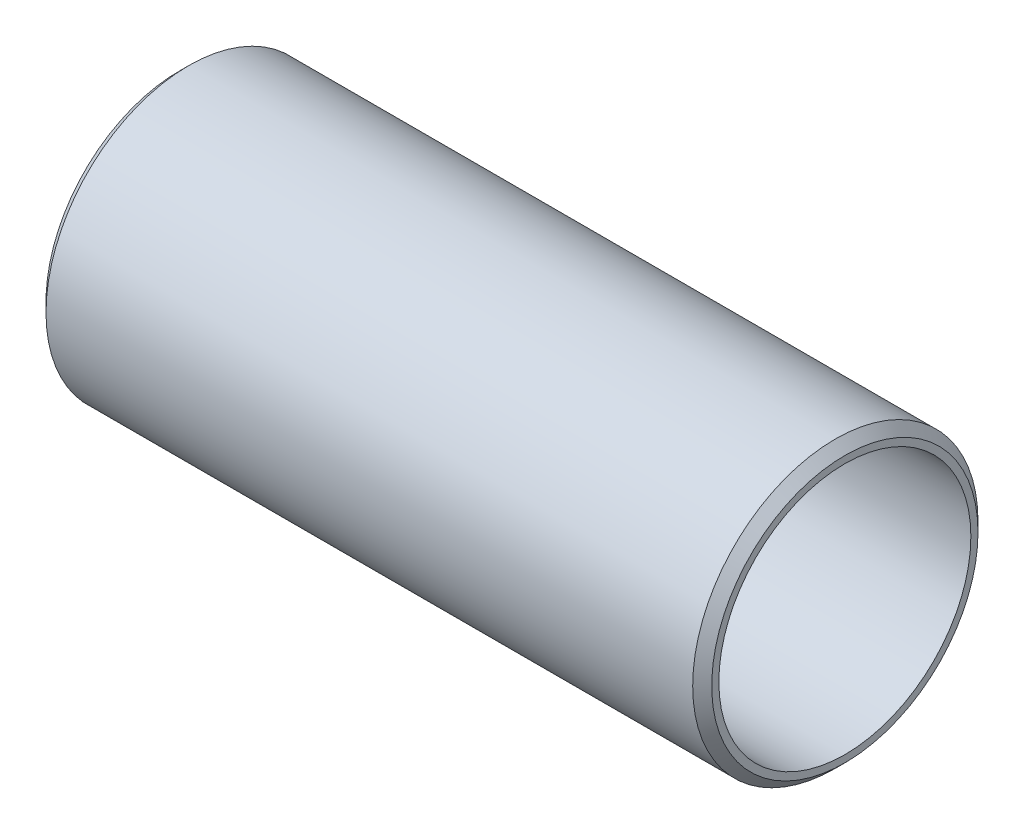
SolidWorks part; units mm, degrees
material "镀锌焊接钢管 Q215A"
ref_plane "前视基准面" through (0, 0, 0) normal (0, 0, 1) x (1, 0, 0)
ref_plane "上视基准面" through (0, 0, 0) normal (0, 1, 0) x (1, 0, 0)
ref_plane "右视基准面" through (0, 0, 0) normal (1, 0, 0) x (0, 0, -1)
sketch "草图1" plane through (0, 0, 0) normal (1, 0, 0) x (0, 0, -1)
  circle A0 centre (0, 0) radius 30
  dimension "D1" = 60
extrude "拉伸-薄壁1" add sketch "草图1" along normal blind 140 thin thin type one direction reverse wall 3.5
cosmetic thread "装饰螺纹线1" parameters "D1"=30, "D2"=56.656
cosmetic thread "装饰螺纹线2" parameters "D1"=30, "D2"=56.656
chamfer "倒角1" distance 2 angle 45 2 edges at (140, 0, -30) (0, 0, -30)
